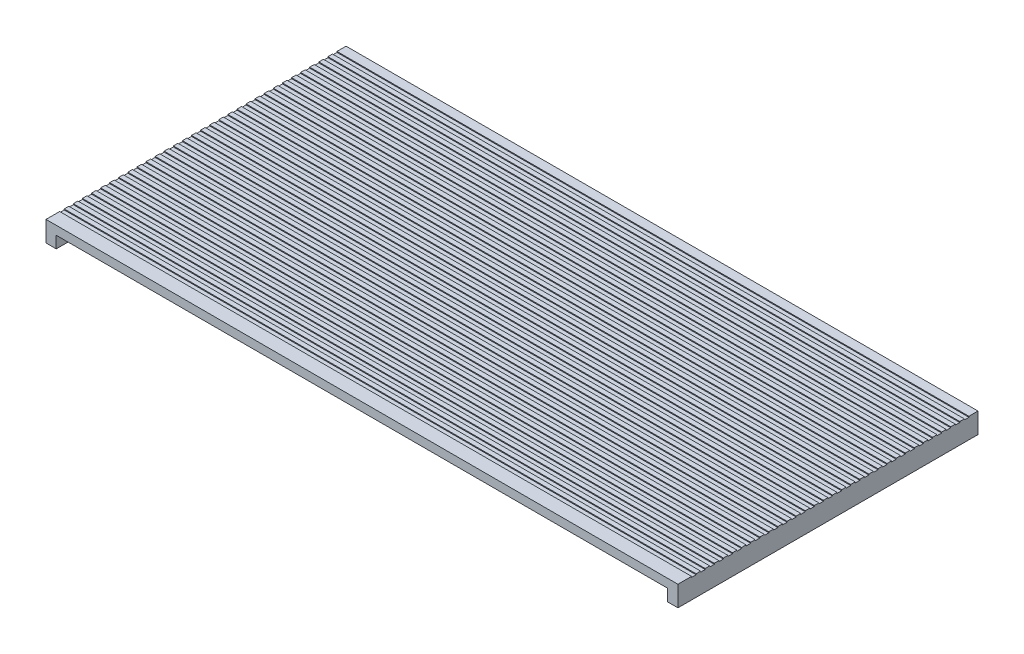
from build123d import *

# Parameters (mm, degrees)
BOSS_EXTRUDE1_DEPTH = 660
SKETCH2_W           = 1390
SKETCH2_H           = 10
CUT_EXTRUDE1_DEPTH  = 2
LPATTERN1_COUNT     = 31
LPATTERN1_PITCH     = 20


with BuildPart() as part:
    # Sketch1 → Boss-Extrude1 (new body)
    with BuildSketch(Plane.XY):
        Polygon((0, 3.5), (0, 22.5), (-695, 22.5), (-695, -22.5), (-672.5, -22.5), (-672.5, 3.5), align=None)
        Polygon((695, 22.5), (0, 22.5), (0, 3.5), (672.5, 3.5), (672.5, -22.5), (695, -22.5), align=None)
    extrude(amount=BOSS_EXTRUDE1_DEPTH)

    # Sketch2 → Cut-Extrude1 (cut)
    with BuildSketch(Plane(origin=(0, 22.5, 0), x_dir=(1, 0, 0), z_dir=(0, 1, 0))):
        with Locations((0, -25)):
            Rectangle(SKETCH2_W, SKETCH2_H)
    cut_extrude1 = extrude(amount=-CUT_EXTRUDE1_DEPTH, mode=Mode.SUBTRACT)

    # LPattern1: Cut-Extrude1 ×31
    with Locations(*[(0, 0, i * LPATTERN1_PITCH) for i in range(1, LPATTERN1_COUNT)]):
        add(cut_extrude1, mode=Mode.SUBTRACT)


solid = part.part
